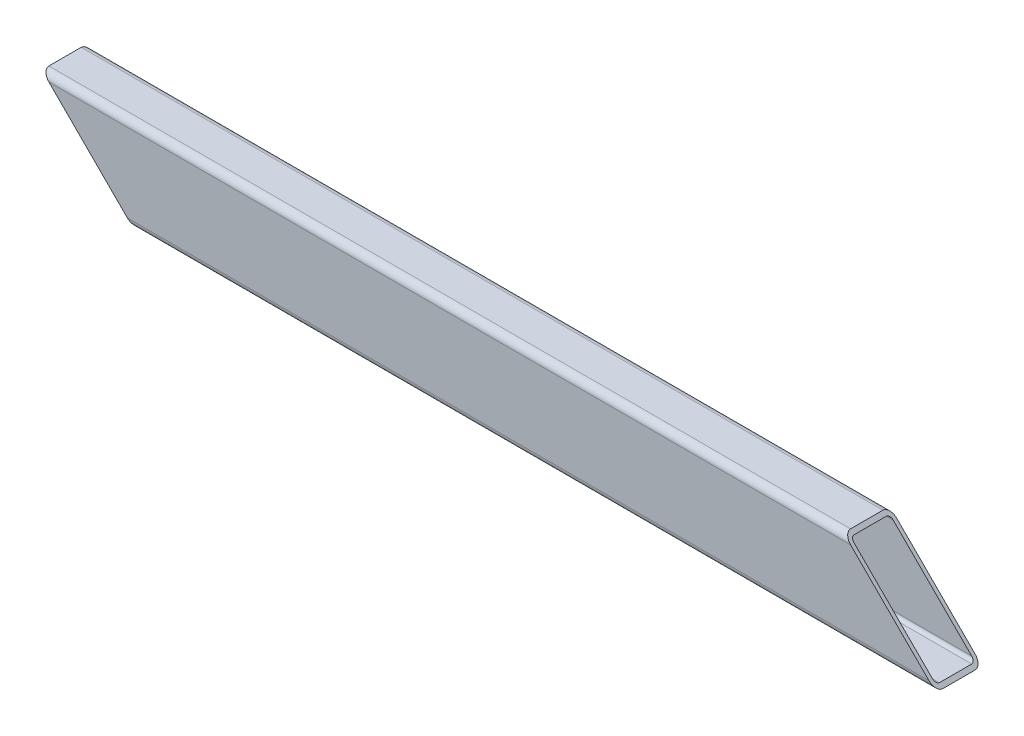
SolidWorks part; units mm, degrees
material "45#"
ref_plane "Front Plane" through (0, 0, 0) normal (0, 0, 1) x (1, 0, 0)
ref_plane "Top Plane" through (0, 0, 0) normal (0, 1, 0) x (1, 0, 0)
ref_plane "Right Plane" through (0, 0, 0) normal (1, 0, 0) x (0, 0, -1)
sketch3d "3DSketch1"
  line L0 (0, 0, 0) -> (775, 0, 0)
  dimension "D1" = 775
other "Cold-Formed Rect Hollow Section GB/T 6728-2002 80 X 40 X 3(1)"
ref_plane "Plane1" through (0, 0, 0) normal (1, 0, 0) x (0, 0, -1)
sketch "Sketch1" plane through (0, 0, 0) normal (1, 0, 0) x (0, 0, -1)
  line L0 (-14, -37) -> (14, -37)
  line L1 (-17, -34) -> (-17, 34)
  line L2 (14, 37) -> (-14, 37)
  line L3 (17, 34) -> (17, -34)
  line L4 (-14, -40) -> (14, -40)
  line L5 (-20, -34) -> (-20, 34)
  line L6 (14, 40) -> (-14, 40)
  line L7 (20, 34) -> (20, -34)
  arc A0 (20, 34) -> (14, 40) centre (14, 34) ccw
  arc A1 (14, -40) -> (20, -34) centre (14, -34) ccw
  arc A2 (-20, -34) -> (-14, -40) centre (-14, -34) ccw
  arc A3 (-14, 40) -> (-20, 34) centre (-14, 34) ccw
  arc A4 (-14, 37) -> (-17, 34) centre (-14, 34) ccw
  arc A5 (17, 34) -> (14, 37) centre (14, 34) ccw
  arc A6 (14, -37) -> (17, -34) centre (14, -34) ccw
  arc A7 (-17, -34) -> (-14, -37) centre (-14, -34) ccw
  point P0 (0, 40)
  point P1 (20, 0)
  point P2 (0, -40)
  point P3 (-20, 0)
  point P4 (-20, 40)
  point P5 (20, 40)
  point P6 (20, -40)
  point P7 (-20, -40)
  point P8 (0, 0)
  point P33 (0, 0)
  dimension "D1" = 6
  dimension "Thickness" = 3
  dimension "V_leg" = 80
  dimension "H_leg" = 40
sketch "Sketch2" plane through (0, 0, 20) normal (0, 0, 1) x (1, 0, 0)
  line L0 (0, 40) -> (80, -40)
  line L1 (0, -40) -> (80, -40)
  line L5 (0, -34) -> (0, -40) construction
  line L7 (0, 34) -> (0, -34) construction
  line L8 (0, 40) -> (0, 34) construction
  line L9 (775, 40) -> (695, 40)
  line L10 (775, 40) -> (0, 40) construction
  line L11 (695, 40) -> (775, -40)
  line L12 (0, -34) -> (0, -40)
  line L13 (775, -40) -> (0, -40) construction
  line L14 (0, 34) -> (0, -34)
  line L15 (0, 40) -> (0, 34)
  line L16 (775, -40) -> (775, 40)
  dimension "D1" = 45
  dimension "D2" = 45
extrude "Cut-Extrude1" cut sketch "Sketch2" against normal through all
